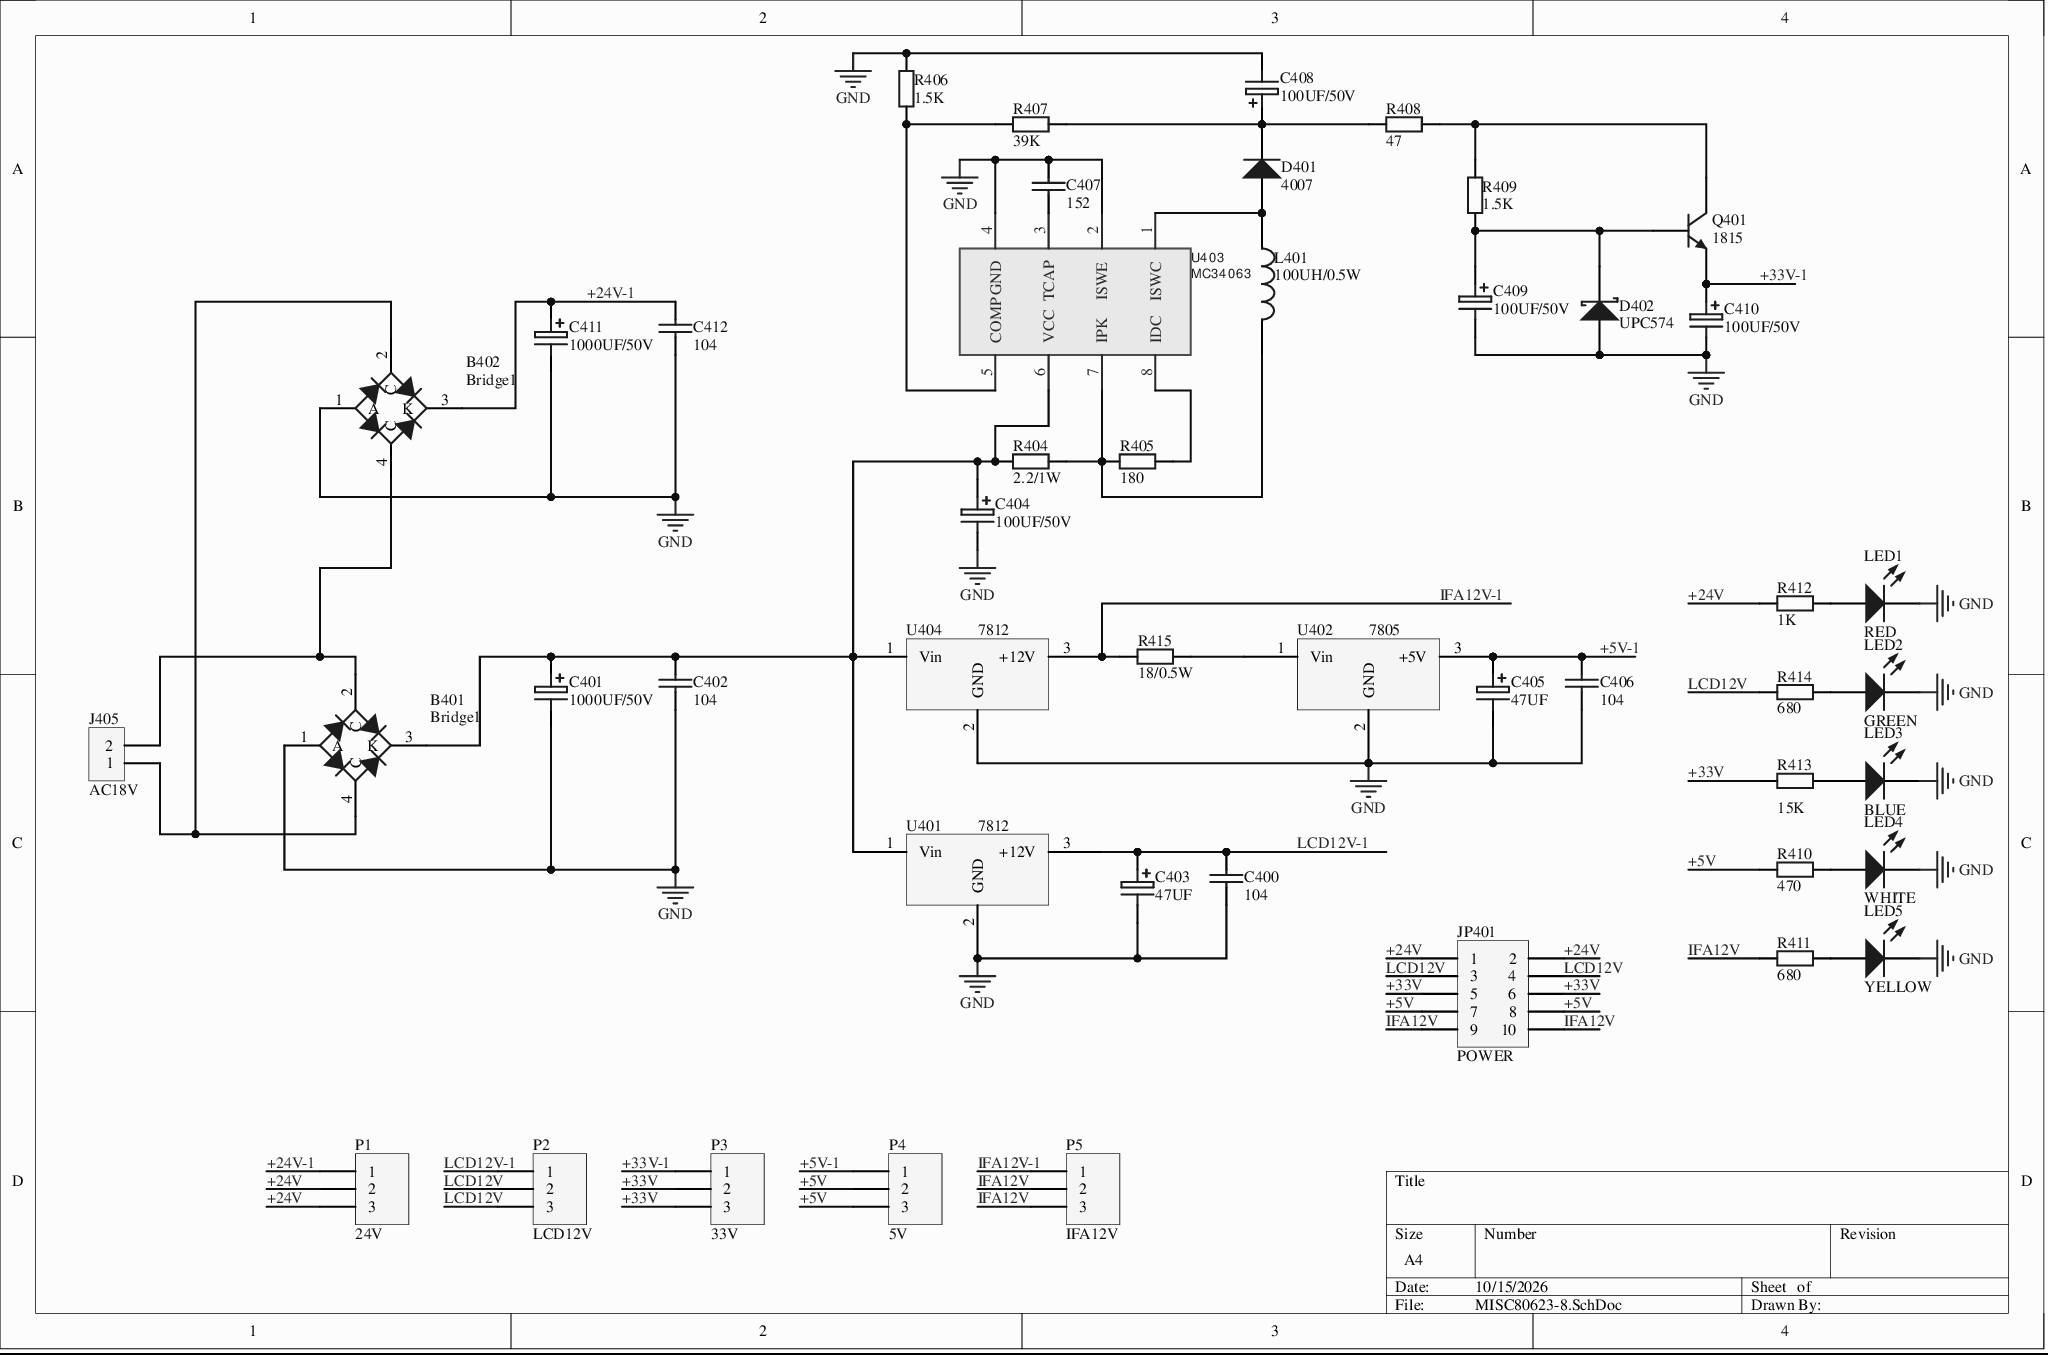
[diagram p0: MISC80623-8.SchDoc]
# Altium project MISC80623-3.PrjPcb
1 sheet, 47 parts. Net scope: global (net labels, ports and power ports of the same name join across sheets).
Board file: MISC80623.PcbDoc

## Sheet MISC80623-8.SchDoc
size A4

### Parts
B401  Bridge1  [B401]
B402  Bridge1  [B401]
C400  104  [DR]
C401  1000UF/50V  [C401]
C402  104  [DR]
C403  47UF  [C401]
C404  100UF/50V  [C401]
C405  47UF  [C401]
C406  104  [DR]
C407  152  [DR]
C408  100UF/50V  [C401]
C409  100UF/50V  [C401]
C410  100UF/50V  [C401]
C411  1000UF/50V  [C401]
C412  104  [DR]
D401  4007  [DO-35]
D402  UPC574  [DO-204AL]
J405  AC18V  [J405]
JP401  POWER  [JP401]
L401  100UH/0.5W  [AL0204]
LED1  RED  [LED]
LED2  GREEN  [LED]
LED3  BLUE  [LED]
LED4  WHITE  [LED]
LED5  YELLOW  [LED]
P1  24V  [HDR1X3]
P2  LCD12V  [HDR1X3]
P3  33V  [HDR1X3]
P4  5V  [HDR1X3]
P5  IFA12V  [HDR1X3]
Q401  1815  [Q401]
R404  2.2/1W  [AXIAL-0.4]
R405  180  [AXIAL-0.4]
R406  1.5K  [AXIAL-0.4]
R407  39K  [AXIAL-0.4]
R408  47  [AXIAL-0.4]
R409  1.5K  [AXIAL-0.4]
R410  470  [AXIAL-0.4]
R411  680  [AXIAL-0.4]
R412  1K  [AXIAL-0.4]
R413  15K  [AXIAL-0.4]
R414  680  [AXIAL-0.4]
R415  18/0.5W  [AXIAL-0.4]
U401  7812  [U404]
U402  7805  [U404]
U403  MC34063  [MC34063]
U404  7812  [U404]

### Nets
GND: B401.1(A) B402.1(A) C400.1 C401.2 C402.1 C403.2 C404.2 C405.2 C406.1 C407.2 C408.2 C409.2 C410.2 C411.2 C412.1 D402.1(A) LED1.2(K) LED2.2(K) LED3.2(K) LED4.2(K) LED5.2(K) R406.2 U401.2(GND) U402.2(GND) U403.2(ISWE) U403.4(GND) U404.2(GND)
+5V: JP401.7 JP401.8 P4.2 P4.3 R410.1
+5V-1: C405.1 C406.2 P4.1 U402.3(+5V)
+24V: JP401.1 JP401.2 P1.2 P1.3 R412.1
+24V-1: B402.3(K) C411.1 C412.2 P1.1
+33V: JP401.5 JP401.6 P3.2 P3.3 R413.1
+33V-1: C410.1 P3.1 Q401.1(E)
IFA12V: JP401.9 JP401.10 P5.2 P5.3 R411.1
IFA12V-1: P5.1 R415.1 U404.3(+12V)
LCD12V: JP401.3 JP401.4 P2.2 P2.3 R414.1
LCD12V-1: C400.2 C403.1 P2.1 U401.3(+12V)
NetB401_2: B401.2(C) B402.4(C) J405.2
NetB401_3: B401.3(K) C401.1 C402.2 C404.1 R404.1 U401.1(Vin) U403.6(VCC) U404.1(Vin)
NetB401_4: B401.4(C) B402.2(C) J405.1
NetC407_1: C407.1 U403.3(TCAP)
NetC408_1: C408.1 D401.2(K) R407.2 R408.1
NetC409_1: C409.1 D402.2(K) Q401.2(B) R409.1
NetD401_1: D401.1(A) L401.1 U403.1(ISWC)
NetL401_2: L401.2 R404.2 R405.1 U403.7(IPK)
NetLED1_1: LED1.1(A) R412.2
NetLED2_1: LED2.1(A) R414.2
NetLED3_1: LED3.1(A) R413.2
NetLED4_1: LED4.1(A) R410.2
NetLED5_1: LED5.1(A) R411.2
NetQ401_3: Q401.3(C) R408.2 R409.2
NetR405_2: R405.2 U403.8(IDC)
NetR406_1: R406.1 R407.1 U403.5(COMP)
NetR415_2: R415.2 U402.1(Vin)

### Library data of the parts
B401 B402 = Bridge1: Full Wave Diode Bridge; Published: 8-Jun-2000; LatestRevisionDate: 29-May-2009; LatestRevisionNote: Sch pins A & K swapped.; DatasheetVersion: E2732B; PackageReference: D-38; PackageDescription: Bridge Rectifier; 4 Terminals; Body 9.4 x 9.4 mm (typ); Pitch 5.08 mm; Publisher: Altium Limited
C400 C402 C406 C407 C412 = CAP
C401 C403-C405 C408-C411 = ELECTRO1
D401 = Diode 1N4448: High Conductance Fast Diode; Published: 8-Jun-2000; LatestRevisionDate: 17-Jul-2002; LatestRevisionNote: Re-released for DXP Platform.; DatasheetVersion: 1997; PackageReference: DO-35; PackageDescription: Diode, Axial; Body 3.8 x 1.9 mm (LxDia. max), Lead Dia. 0.53 mm (max); Code_JEDEC: DO-204-AH; ComponentLink1Description: Manufacturer Link; ComponentLink2Description: Datasheet; ComponentLink2URL: http://www.fairchildsemi.com/ds/1N%2F1N4448.pdf; Publisher: Altium Limited
D402 = Diode 11DQ03: Schottky Rectifier; Published: 8-Jun-2000; LatestRevisionDate: 17-Jul-2002; LatestRevisionNote: Re-released for DXP Platform.; DatasheetVersion: Dec-1997; PackageReference: DO-204AL; PackageDescription: Diode, Axial; Body 5.2 x 2.7 mm (LxDia. max), Lead Dia. 0.86 mm (max); Code_JEDEC: DO-204-AL; ComponentLink1Description: Manufacturer Link; ComponentLink2Description: Datasheet; ComponentLink2URL: http://www.irf.com/product-info/datasheets/data/11dq03.pdf; Publisher: Altium Limited
J405 = Header 2: Header, 2-Pin; LatestRevisionDate: 17-Jul-2002; LatestRevisionNote: Re-released for DXP Platform.; Publisher: Altium Limited
JP401 = Header 5X2: Header, 5-Pin, Dual row; LatestRevisionDate: 17-Jul-2002; LatestRevisionNote: Re-released for DXP Platform.; Publisher: Altium Limited
L401 = INDUCTOR
LED1-LED5 = LED0: Typical INFRARED GaAs LED; Published: 8-Jun-2000; LatestRevisionDate: 08-Jul-2005; LatestRevisionNote: Mech Layer 1 removed.; PackageReference: LED-0; PackageDescription: LED; 2 Leads; Publisher: Altium Limited
P1-P5 = Header 3: Header, 3-Pin; LatestRevisionDate: 17-Jul-2002; LatestRevisionNote: Re-released for DXP Platform.; Publisher: Altium Limited
Q401 = 2N3904: NPN General Purpose Amplifier; Published: 8-Jun-2000; LatestRevisionDate: 15-Jan-2003; LatestRevisionNote: PCB Footprint 'BCY-W3/D4.7' replaced; DatasheetVersion: 1997; PackageVersion: Sep-1998; PackageReference: TO-92A; PackageDescription: TO, Flat Index; 3 In-Line, Axial Leads; Body Dia. 4.5mm; Leads 0.51 x 0.48 mm (max); ComponentLink1Description: Manufacturer Link; ComponentLink2Description: Datasheet; ComponentLink2URL: http://www.fairchildsemi.com/ds/2N%2F2N3904.pdf; Publisher: Altium Limited
R404-R411 R413-R415 = Res2: Resistor; Value: 1K; Published: 8-Jun-2000; LatestRevisionDate: 17-Jul-2002; LatestRevisionNote: Re-released for DXP Platform.; PackageReference: AXIAL-0.4; PackageDescription: Axial Device, Thru-Hole; 2 Leads; 0.4 in Pin Spacing; Publisher: Altium Limited
R412 = Res2: Resistor; Published: 8-Jun-2000; LatestRevisionDate: 17-Jul-2002; LatestRevisionNote: Re-released for DXP Platform.; PackageReference: AXIAL-0.4; PackageDescription: Axial Device, Thru-Hole; 2 Leads; 0.4 in Pin Spacing; Value: 1K; Publisher: Altium Limited
U401 U402 U404 = AMS1117: three-terminal voltage regulator